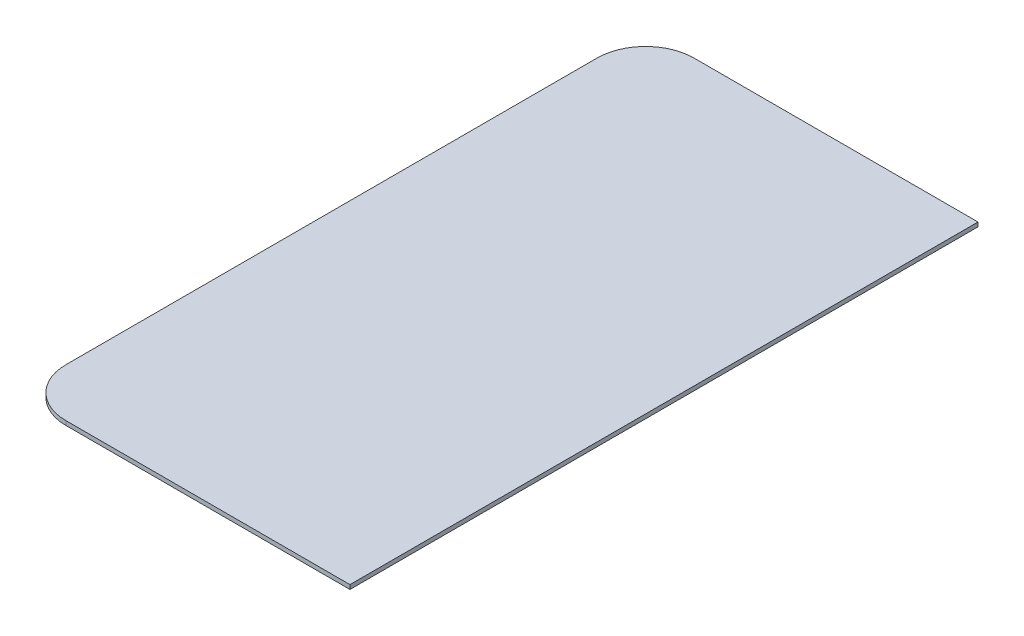
from build123d import *

# Parameters (mm, degrees)
BOSS_EXTRUDE1_DEPTH = 4


with BuildPart() as part:
    # Sketch1 → Boss-Extrude1 (new body)
    with BuildSketch(Plane(origin=(0, 0, 0), x_dir=(1, 0, 0), z_dir=(0, 1, 0))):
        with BuildLine():
            Line((0, 298), (-269.5, 298))
            ThreePointArc((-269.5, 298), (-302.026911935, 284.526911935), (-315.5, 252))
            Line((-315.5, 252), (-315.5, -252))
            ThreePointArc((-315.5, -252), (-302.026911935, -284.526911935), (-269.5, -298))
            Line((-269.5, -298), (0, -298))
            Line((0, -298), (0, 298))
        make_face()
    extrude(amount=BOSS_EXTRUDE1_DEPTH)


solid = part.part
